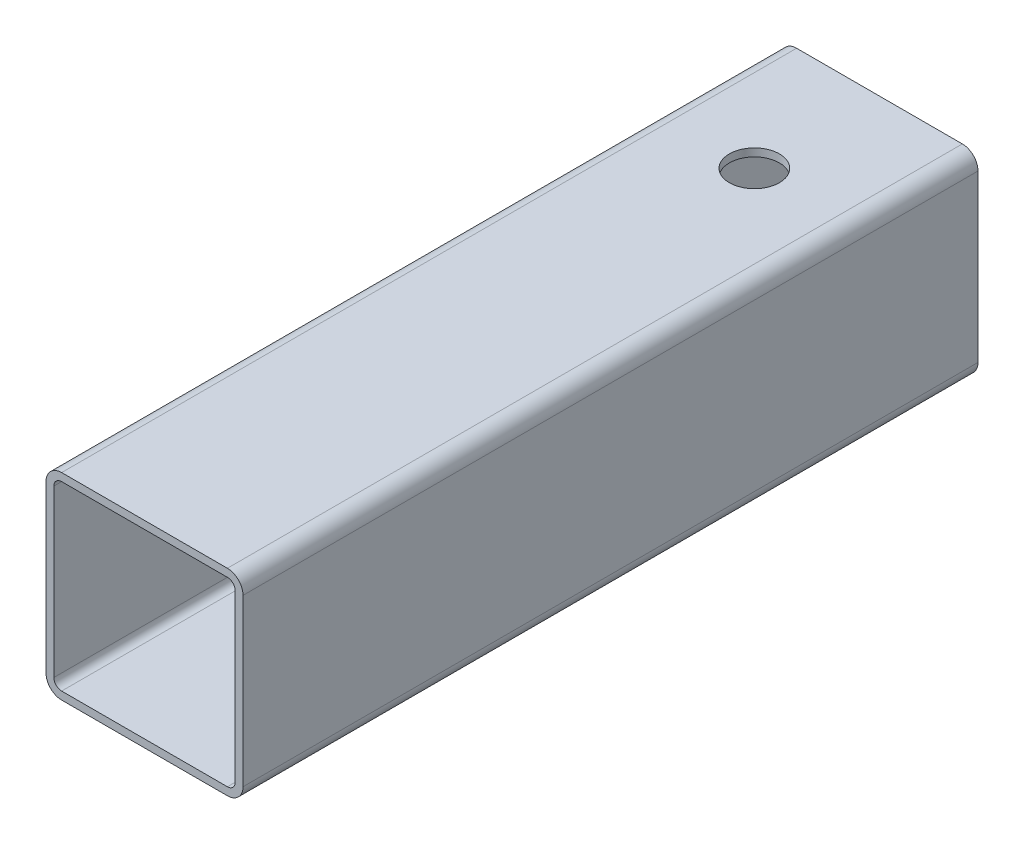
SolidWorks part; units mm, degrees
material "Q235A"
ref_plane "Plane1" through (0, 0, 0) normal (0, 0, 1) x (1, 0, 0)
ref_plane "Plane2" through (0, 0, 0) normal (0, 1, 0) x (1, 0, 0)
ref_plane "Plane3" through (0, 0, 0) normal (1, 0, 0) x (0, 0, -1)
sketch "Sketch1" plane through (0, 0, 0) normal (0, 0, 1) x (1, 0, 0)
  line L0 (-53, -58) -> (53, -58)
  line L1 (-58, -53) -> (-58, 53)
  line L2 (53, 58) -> (-53, 58)
  line L3 (58, 53) -> (58, -53)
  line L4 (-53, -63) -> (53, -63)
  line L5 (-63, -53) -> (-63, 53)
  line L6 (53, 63) -> (-53, 63)
  line L7 (63, 53) -> (63, -53)
  arc A0 (63, 53) -> (53, 63) centre (53, 53) ccw
  arc A1 (53, -63) -> (63, -53) centre (53, -53) ccw
  arc A2 (-63, -53) -> (-53, -63) centre (-53, -53) ccw
  arc A3 (-53, 63) -> (-63, 53) centre (-53, 53) ccw
  arc A4 (-53, 58) -> (-58, 53) centre (-53, 53) ccw
  arc A5 (58, 53) -> (53, 58) centre (53, 53) ccw
  arc A6 (53, -58) -> (58, -53) centre (53, -53) ccw
  arc A7 (-58, -53) -> (-53, -58) centre (-53, -53) ccw
  point P0 (-63, 0)
  point P1 (63, 0)
  point P2 (0, 63)
  point P3 (0, -63)
  point P4 (0, 0)
  point P5 (-63, -63)
  point P6 (63, -63)
  point P7 (63, 63)
  point P8 (-63, 63)
extrude "Boss-Extrude1" add sketch "Sketch1" along normal mid plane 470
sketch "草图1" plane through (0, 0, 0) normal (0, 1, 0) x (1, 0, 0)
  line L0 (53, 235) -> (-53, 235) construction
  circle A0 centre (0, 155) radius 16
  dimension "D2" = 32
  dimension "D1" = 80
extrude "Cut-Extrude1" cut sketch "草图1" against normal through all both and the other way through all
